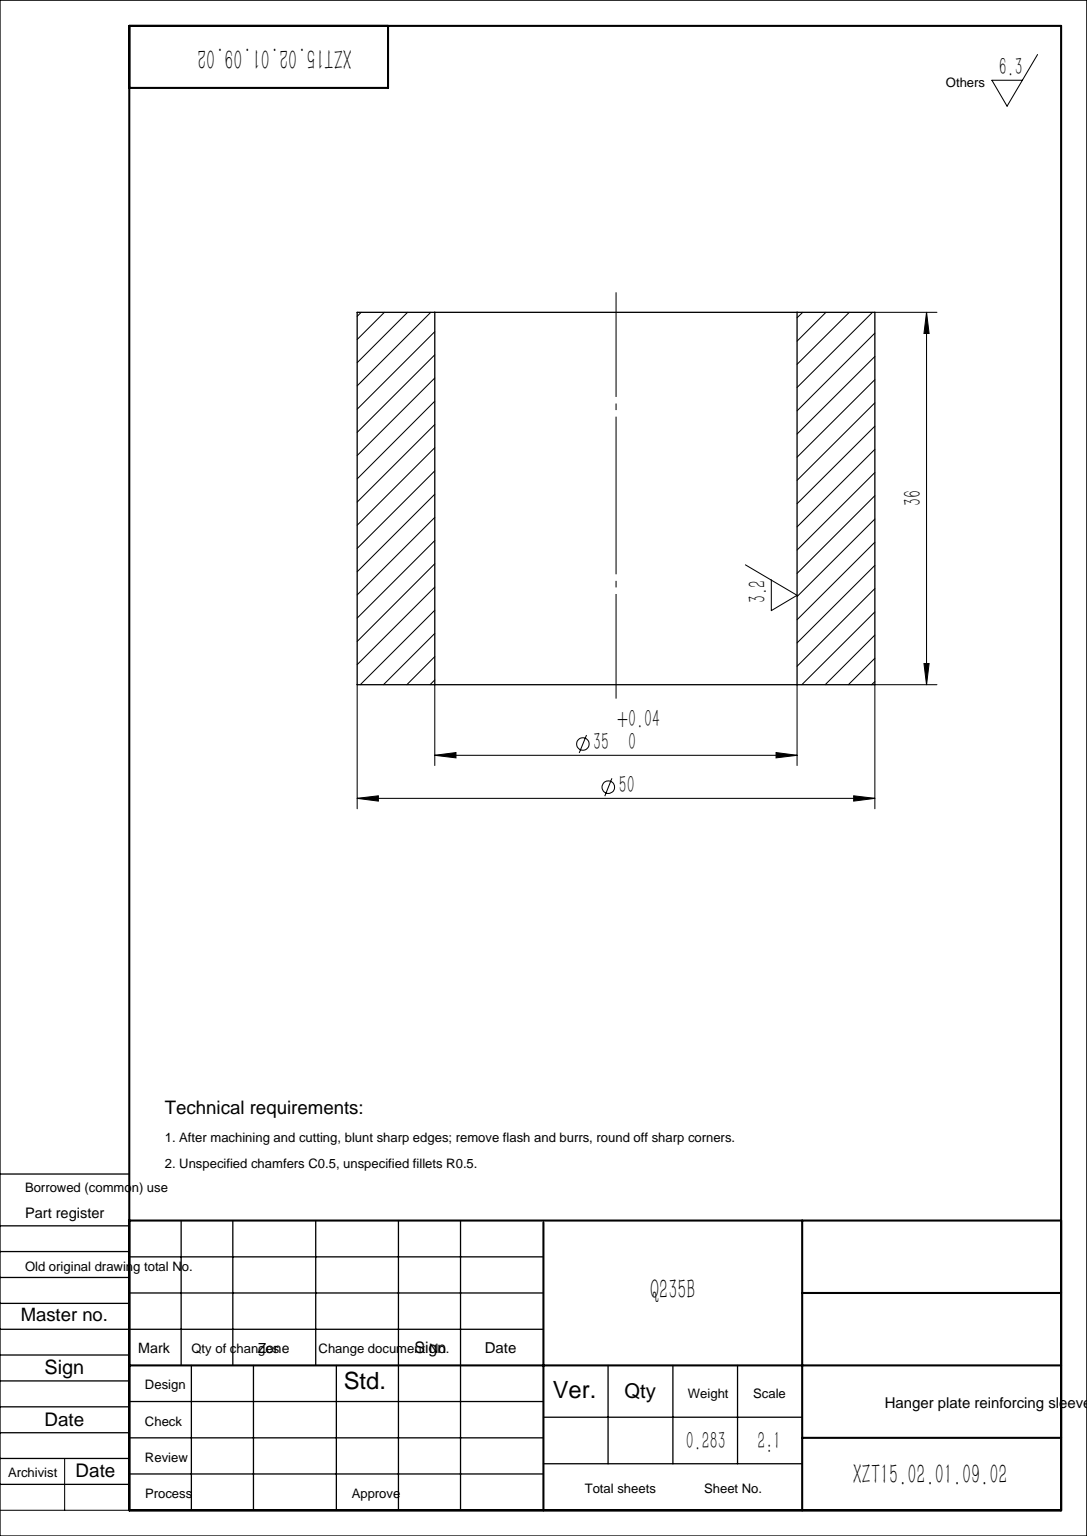
from build123d import *

# Parameters (mm, degrees)
SKETCH1_R           = 25
SKETCH1_R_2         = 17.5
BOSS_EXTRUDE1_DEPTH = 36


with BuildPart() as part:
    # Sketch1 → Boss-Extrude1 (new body)
    with BuildSketch(Plane(origin=(0, 0, 0), x_dir=(1, 0, 0), z_dir=(0, 1, 0))):
        with Locations(Location((0, 0, 0), (0, 0, 270))):
            Circle(SKETCH1_R)
        with Locations(Location((0, 0, 0), (0, 0, 270))):
            Circle(SKETCH1_R_2, mode=Mode.SUBTRACT)
    extrude(amount=BOSS_EXTRUDE1_DEPTH)


solid = part.part
